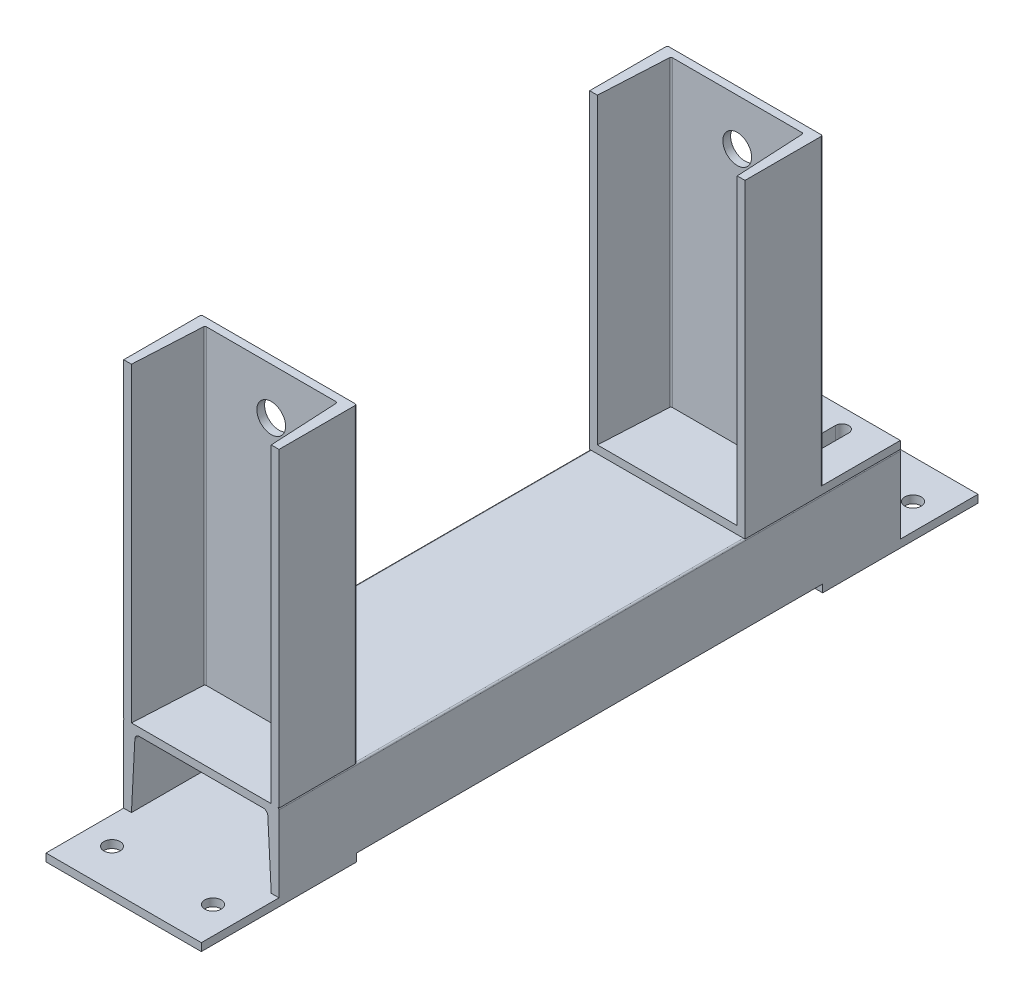
SolidWorks part; units mm, degrees
material "1060 Alloy"
ref_plane "Front Plane" through (0, 0, 0) normal (0, 0, 1) x (1, 0, 0)
ref_plane "Top Plane" through (0, 0, 0) normal (0, 1, 0) x (1, 0, 0)
ref_plane "Right Plane" through (0, 0, 0) normal (1, 0, 0) x (0, 0, -1)
sketch "Sketch1" plane through (0, 0, 0) normal (0, 0, 1) x (1, 0, 0)
  line L0 (0, 0) -> (0, 49)
  line L1 (1, 50) -> (99, 50)
  line L2 (100, 49) -> (100, 0)
  line L3 (100, 0) -> (95, 0)
  line L4 (95, 0) -> (92.7906, 42.157)
  line L5 (89.7948, 45) -> (10.2052, 45)
  line L6 (7.2094, 42.157) -> (5, 0)
  line L7 (5, 0) -> (0, 0)
  arc A0 (92.7906, 42.157) -> (89.7948, 45) centre (89.7948, 42) ccw
  arc A1 (7.2094, 42.157) -> (10.2052, 45) centre (10.2052, 42) cw
  arc A2 (100, 49) -> (99, 50) centre (99, 49) ccw
  arc A3 (0, 49) -> (1, 50) centre (1, 49) cw
  point P3 (0, 0)
  point P10 (0, 0)
  point P17 (100, 50)
  point P20 (0, 50)
  dimension "D8" = 3
  dimension "D9" = 1
  dimension "D1" = 50
  dimension "D2" = 100
  dimension "D3" = 5
  dimension "D4" = 5
  dimension "D5" = 5
  dimension "D6" = 3
  dimension "D7" = 3
extrude "Boss-Extrude1" add sketch "Sketch1" along normal blind 400
sketch "Sketch2" plane through (0, 0, 0) normal (0, -1, 0) x (1, 0, 0)
  line L0 (100, 400) -> (100, 0) construction
  line L1 (100, 350) -> (0, 350)
  line L2 (100, 350) -> (100, 450)
  line L3 (100, 450) -> (0, 450)
  line L4 (0, 350) -> (0, 450)
  line L5 (10.2052, 400) -> (89.7948, 400) construction
  line L6 (10.2052, 0) -> (89.7948, 0) construction
  line L7 (100, 50) -> (0, 50)
  line L8 (100, 50) -> (100, -50)
  line L9 (100, -50) -> (0, -50)
  line L10 (0, 50) -> (0, -50)
  dimension "D1" = 100
  dimension "D2" = 50
  dimension "D3" = 100
  dimension "D4" = 100
  dimension "D5" = 50
  dimension "D6" = 100
extrude "Boss-Extrude2" add sketch "Sketch2" along normal blind 5
hole_wizard "Ø10.5 (10.5) Diameter Hole1" positions "Sketch3" profile "Sketch4" hole size "Ø10.5" standard "ISO" end condition through all
sketch "Sketch3" plane through (0, 0, 0) normal (0, 1, 0) x (1, 0, 0)
  line L0 (0, 50) -> (100, 50) construction
  line L1 (100, -450) -> (0, -450) construction
  line L2 (0, -450) -> (0, -400) construction
  point P0 (17.5, -425)
  point P2 (82.5, -425)
  point P4 (83.1487, 25)
  point P6 (17.5, 25)
  point P13 (0, 0)
  point P14 (0, 0)
  point P15 (0, 0)
  point P16 (0, 0)
  dimension "D1" = 25
  dimension "D2" = 25
  dimension "D3" = 65
  dimension "D4" = 17.5
sketch "Sketch4" plane through (17.5, 0, 425) normal (1, 0, 0) x (0, 0, 1)
  line L0 (0, 0) -> (0, 5)
  line L1 (0, 5) -> (5.25, 5)
  line L2 (5.25, 5) -> (5.25, 0)
  line L5 (5.25, 0) -> (0, 0)
  line L11 (0, -6.35) -> (0, 107.95) construction
  dimension "Thru Hole Dia." = 10.5
  dimension "Thru Hole Depth" = 5
sketch "Sketch5" plane through (0, 50, 0) normal (0, 1, 0) x (1, 0, 0)
  line L0 (1, -350) -> (99, -350)
  line L1 (100, -400) -> (100, 0) construction
  line L2 (100, -351) -> (100, -400)
  line L3 (100, -400) -> (95, -400)
  line L4 (95, -400) -> (92.6913, -355.9477)
  line L5 (91.6927, -355) -> (8.3073, -355)
  line L6 (7.3087, -355.9477) -> (5, -400)
  line L7 (99, -400) -> (1, -400) construction
  line L8 (5, -400) -> (0, -400)
  line L9 (0, -400) -> (0, -351)
  arc A0 (1, -350) -> (0, -351) centre (1, -351) ccw
  arc A1 (100, -351) -> (99, -350) centre (99, -351) ccw
  arc A2 (92.6913, -355.9477) -> (91.6927, -355) centre (91.6927, -356) ccw
  arc A3 (8.3073, -355) -> (7.3087, -355.9477) centre (8.3073, -356) ccw
  point P7 (0, 0)
  point P16 (0, 0)
  point P19 (0, -350)
  point P22 (100, -350)
  dimension "D6" = 1
  dimension "D1" = 5
  dimension "D2" = 5
  dimension "D3" = 3
  dimension "D4" = 5
  dimension "D5" = 3
extrude "Boss-Extrude3" add sketch "Sketch5" along normal blind 200 contours L6 L8 L9 A0 L0 A1 L2 L3 L4 A2 L5 A3
sketch "Sketch6" plane through (0, 50, 0) normal (0, 1, 0) x (1, 0, 0)
  line L0 (100, -400) -> (100, 0) construction
  line L1 (0, 0) -> (100, 0)
  line L2 (0, 0) -> (0, -100)
  line L3 (0, -100) -> (100, -100)
  line L4 (100, 0) -> (100, -100)
  dimension "D1" = 100
extrude "Boss-Extrude4" add sketch "Sketch6" along normal blind 5
sketch "Sketch7" plane through (0, 55, 0) normal (0, 1, 0) x (1, 0, 0)
  line L0 (1, -50) -> (99, -50)
  line L1 (100, -100) -> (100, 0) construction
  line L2 (100, -51) -> (100, -100)
  line L3 (100, -100) -> (95, -100)
  line L4 (1, -100) -> (99, -100) construction
  line L5 (95, -100) -> (92.6913, -55.9477)
  line L6 (91.6927, -55) -> (8.3073, -55)
  line L7 (7.3087, -55.9477) -> (5, -100)
  line L8 (0, -100) -> (100, -100) construction
  line L9 (5, -100) -> (0, -100)
  line L10 (0, -100) -> (0, -51)
  arc A0 (100, -51) -> (99, -50) centre (99, -51) ccw
  arc A1 (1, -50) -> (0, -51) centre (1, -51) ccw
  arc A2 (92.6913, -55.9477) -> (91.6927, -55) centre (91.6927, -56) ccw
  arc A3 (8.3073, -55) -> (7.3087, -55.9477) centre (8.3073, -56) ccw
  point P19 (100, -50)
  point P22 (0, -50)
  dimension "D6" = 1
  dimension "D1" = 5
  dimension "D2" = 5
  dimension "D3" = 3
  dimension "D4" = 3
  dimension "D5" = 5
extrude "Boss-Extrude5" add sketch "Sketch7" along normal blind 195
sketch "Sketch8" plane through (0, 50, 0) normal (0, 1, 0) x (1, 0, 0)
  line L2 (25, -37.5) -> (25, -12.5) construction
  line L3 (20.75, -37.5) -> (20.75, -12.5)
  line L4 (29.25, -37.5) -> (29.25, -12.5)
  line L5 (0, 0) -> (0, -51) construction
  line L6 (100, 0) -> (0, 0) construction
  line L7 (75, -37.5) -> (75, -12.5) construction
  line L8 (70.75, -37.5) -> (70.75, -12.5)
  line L9 (79.25, -37.5) -> (79.25, -12.5)
  line L10 (100, -51) -> (100, 0) construction
  arc A0 (20.75, -37.5) -> (29.25, -37.5) centre (25, -37.5) ccw
  arc A1 (29.25, -12.5) -> (20.75, -12.5) centre (25, -12.5) ccw
  arc A2 (70.75, -37.5) -> (79.25, -37.5) centre (75, -37.5) ccw
  arc A3 (79.25, -12.5) -> (70.75, -12.5) centre (75, -12.5) ccw
  point P1 (25, -25)
  point P13 (75, -25)
  dimension "D1" = 8.5
  dimension "D2" = 25
  dimension "D3" = 12.5
  dimension "D4" = 25
  dimension "D5" = 8.5
  dimension "D6" = 25
  dimension "D7" = 25
  dimension "D8" = 12.5
extrude "Cut-Extrude1" cut sketch "Sketch8" along normal blind 20 and the other way blind 20
hole_wizard "Ø18.5 (18.5) Diameter Hole1" positions "Sketch9" profile "Sketch10" hole size "Ø18.5" standard "ISO" end condition through all
sketch "Sketch9" plane through (0, 0, 50) normal (0, 0, -1) x (-1, 0, 0)
  line L0 (0, 250) -> (0, 55) construction
  line L1 (-100, 55) -> (0, 55) construction
  point P0 (-50, 220)
  dimension "D1" = 50
  dimension "D2" = 165
sketch "Sketch10" plane through (50, 220, 50) normal (1, 0, 0) x (0, 1, 0)
  line L0 (0, 0) -> (0, 400)
  line L1 (0, 400) -> (9.25, 400)
  line L2 (9.25, 400) -> (9.25, 0)
  line L5 (9.25, 0) -> (0, 0)
  line L11 (0, -6.35) -> (0, 107.95) construction
  dimension "Thru Hole Dia." = 18.5
  dimension "Thru Hole Depth" = 400
